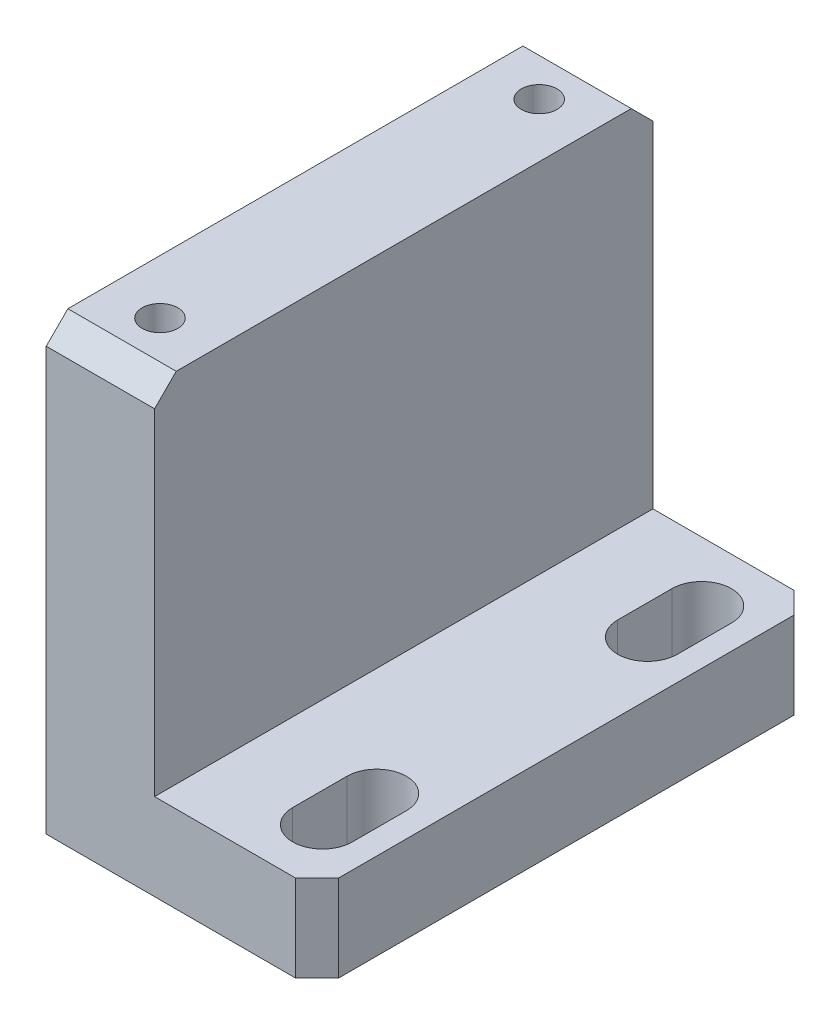
from build123d import *

# Parameters (mm, degrees)
BOSS_EXTRUDE1_DEPTH   = 23
CUT_EXTRUDE1_DEPTH    = 54.244718048
M4_TAPPED_HOLE1_D     = 3.3
M4_TAPPED_HOLE1_DEPTH = 10.1
M4_TAPPED_HOLE1_TIP   = 0.991420021
CHAMFER4_SIZE         = 2


with BuildPart() as part:
    # Sketch1 → Boss-Extrude1 (new, symmetric)
    with BuildSketch(Plane.XY):
        Polygon((0, 41), (10, 41), (10, 8), (25, 8), (25, 0), (0, 0), align=None)
    extrude(amount=BOSS_EXTRUDE1_DEPTH, both=True)

    # Sketch2 → Cut-Extrude1 (cut, through all)
    with BuildSketch(Plane(origin=(0, 0, 0), x_dir=(1, 0, 0), z_dir=(0, 1, 0))):
        with BuildLine():
            Line((22.75, 17.5), (22.75, 12.5))
            ThreePointArc((22.75, 12.5), (20, 9.75), (17.25, 12.5))
            Line((17.25, 12.5), (17.25, 17.5))
            ThreePointArc((17.25, 17.5), (20, 20.25), (22.75, 17.5))
        make_face()
        with BuildLine():
            Line((22.75, -12.5), (22.75, -17.5))
            ThreePointArc((22.75, -17.5), (20, -20.25), (17.25, -17.5))
            Line((17.25, -17.5), (17.25, -12.5))
            ThreePointArc((17.25, -12.5), (20, -9.75), (22.75, -12.5))
        make_face()
    extrude(amount=CUT_EXTRUDE1_DEPTH, mode=Mode.SUBTRACT)

    # M4 Tapped Hole1
    with Locations(Plane(origin=(0, 41, 0), x_dir=(1, 0, 0), z_dir=(0, 1, 0))):
        with Locations((5, 17.5), (5, -17.5)):
            Hole(M4_TAPPED_HOLE1_D / 2, depth=M4_TAPPED_HOLE1_DEPTH)
            with Locations((0, 0, -(M4_TAPPED_HOLE1_DEPTH + M4_TAPPED_HOLE1_TIP / 2))):  # 118° drill point
                Cone(0, M4_TAPPED_HOLE1_D / 2, M4_TAPPED_HOLE1_TIP, mode=Mode.SUBTRACT)

    # Chamfer4
    chamfer4_edges = [part.edges().sort_by_distance(p)[0] for p in [
        (25, 4, 23),
        (5, 41, 23),
        (5, 41, -23),
        (25, 4, -23),
    ]]
    chamfer(chamfer4_edges, length=CHAMFER4_SIZE)


solid = part.part
